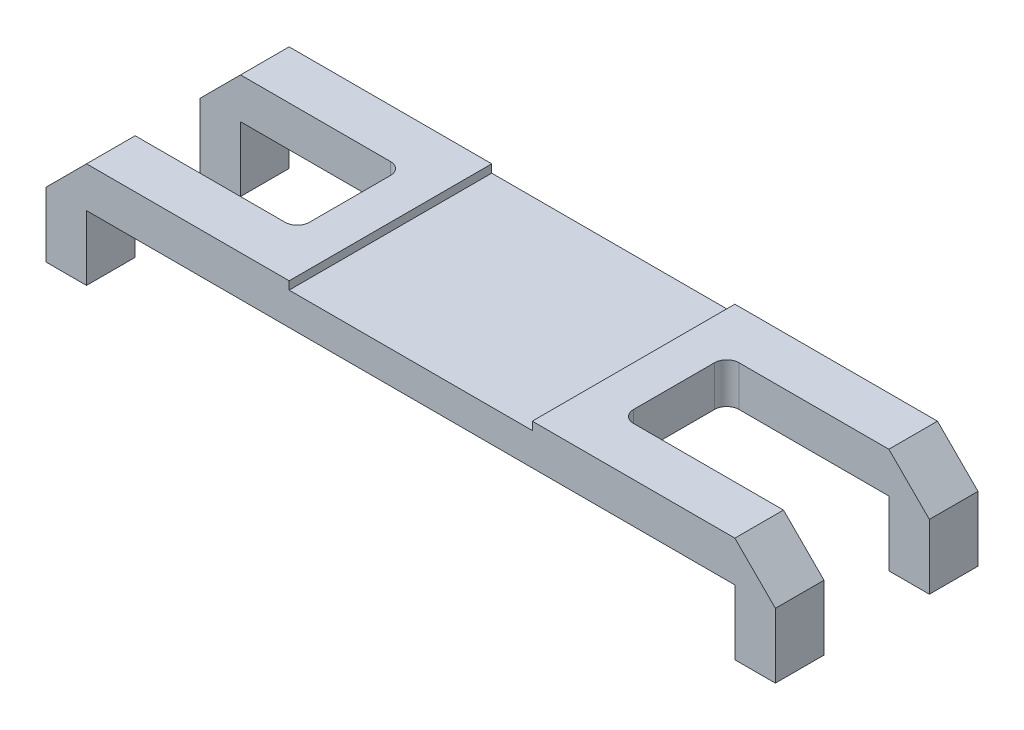
from build123d import *

# Parameters (mm, degrees)
SKETCH1_W           = 180
SKETCH1_H           = 50
BOSS_EXTRUDE1_DEPTH = 10
SKETCH2_W           = 10
SKETCH2_H           = 50
BOSS_EXTRUDE2_DEPTH = 16
SKETCH3_W           = 50
SKETCH3_H           = 26
CUT_EXTRUDE1_DEPTH  = 97.958754117
FILLET1_R           = 3
CHAMFER1_SIZE       = 10
SKETCH4_W           = 60
SKETCH4_H           = 50
CUT_EXTRUDE2_DEPTH  = 2


with BuildPart() as part:
    # Sketch1 → Boss-Extrude1 (new body)
    with BuildSketch(Plane(origin=(0, 0, 0), x_dir=(1, 0, 0), z_dir=(0, 1, 0))):
        Rectangle(SKETCH1_W, SKETCH1_H)
    extrude(amount=BOSS_EXTRUDE1_DEPTH)

    # Sketch2 → Boss-Extrude2 (add)
    with BuildSketch(Plane.XZ):
        with Locations((-85, 0)):
            Rectangle(SKETCH2_W, SKETCH2_H)
        with Locations((85, 0)):
            Rectangle(SKETCH2_W, SKETCH2_H)
    extrude(amount=BOSS_EXTRUDE2_DEPTH)

    # Sketch3 → Cut-Extrude1 (cut, through all)
    with BuildSketch(Plane(origin=(0, 10, 0), x_dir=(1, 0, 0), z_dir=(0, 1, 0))):
        with Locations((-65, 0)):
            Rectangle(SKETCH3_W, SKETCH3_H)
    cut_extrude1 = extrude(amount=-CUT_EXTRUDE1_DEPTH, mode=Mode.SUBTRACT)

    # Mirror1: Cut-Extrude1 across plane
    add(cut_extrude1.mirror(Plane(origin=(0, 0, 0), x_dir=(0, 0, 1), z_dir=(1, 0, 0))), mode=Mode.SUBTRACT)

    # Fillet1
    fillet1_edges = [part.edges().sort_by_distance(p)[0] for p in [
        (-40, 5, -13),
        (-40, 5, 13),
        (40, 5, 13),
        (40, 5, -13),
    ]]
    fillet(fillet1_edges, radius=FILLET1_R)

    # Chamfer1
    chamfer1_edges = [part.edges().sort_by_distance(p)[0] for p in [
        (-90, 10, -19),
        (90, 10, 19),
        (-90, 10, 19),
        (90, 10, -19),
    ]]
    chamfer(chamfer1_edges, length=CHAMFER1_SIZE)

    # Sketch4 → Cut-Extrude2 (cut)
    with BuildSketch(Plane(origin=(0, 10, 0), x_dir=(1, 0, 0), z_dir=(0, 1, 0))):
        Rectangle(SKETCH4_W, SKETCH4_H)
    extrude(amount=-CUT_EXTRUDE2_DEPTH, mode=Mode.SUBTRACT)


solid = part.part
